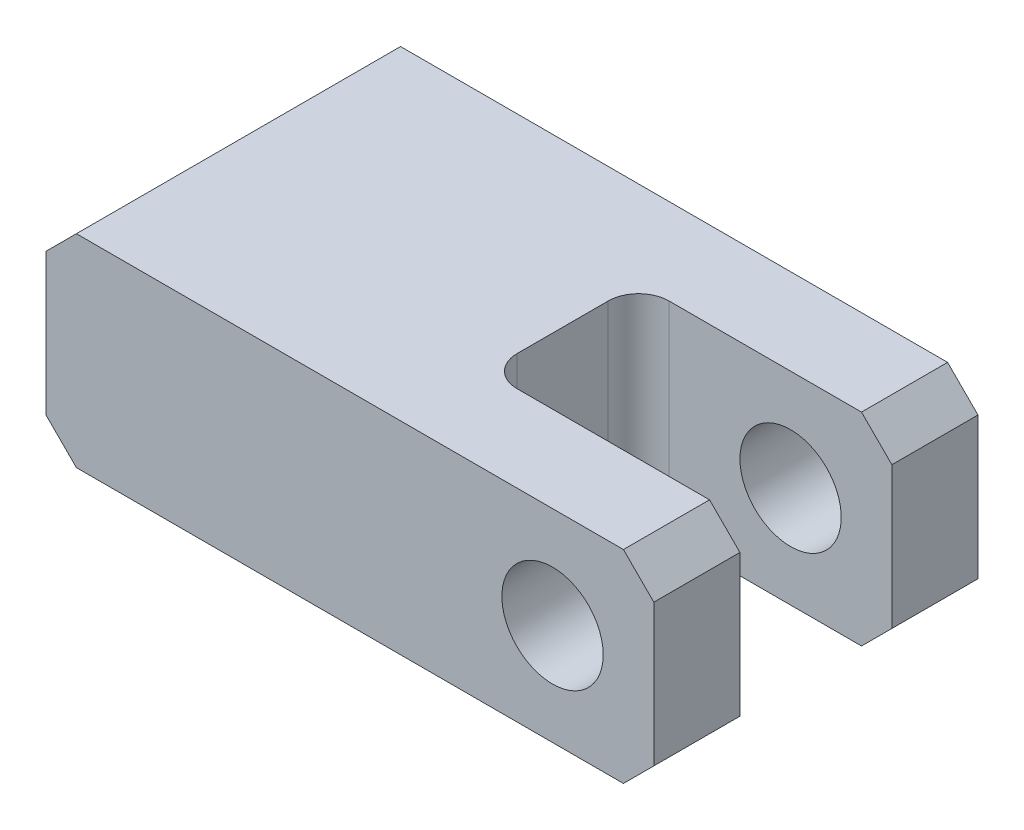
from build123d import *

# Parameters (mm, degrees)
SKETCH1_W             = 60
SKETCH1_H             = 32
BOSS_EXTRUDE1_DEPTH   = 20
SKETCH2_R             = 5
CUT_EXTRUDE1_DEPTH    = 42
CHAMFER1_SIZE         = 3
M6_TAPPED_HOLE1_D     = 5
M6_TAPPED_HOLE1_DEPTH = 15
M6_TAPPED_HOLE1_TIP   = 1.502151548
SKETCH6_W             = 15
SKETCH6_H             = 30
CUT_EXTRUDE2_DEPTH    = 25
FILLET1_R             = 3


with BuildPart() as part:
    # Sketch1 → Boss-Extrude1 (new body)
    with BuildSketch(Plane(origin=(0, 0, 0), x_dir=(1, 0, 0), z_dir=(0, 1, 0))):
        Rectangle(SKETCH1_W, SKETCH1_H)
    extrude(amount=BOSS_EXTRUDE1_DEPTH)

    # Sketch2 → Cut-Extrude1 (cut)
    with BuildSketch(Plane.XY.offset(16)):
        with Locations((20, 10)):
            Circle(SKETCH2_R)
    extrude(amount=-CUT_EXTRUDE1_DEPTH, mode=Mode.SUBTRACT)

    # Chamfer1
    chamfer1_edges = [part.edges().sort_by_distance(p)[0] for p in [
        (30, 20, 0),
        (-30, 20, 0),
        (30, 0, 0),
        (-30, 0, 0),
    ]]
    chamfer(chamfer1_edges, length=CHAMFER1_SIZE)

    # M6 Tapped Hole1
    with Locations(Plane.ZY.offset(30)):
        with Locations((-10, 10), (10, 10)):
            Hole(M6_TAPPED_HOLE1_D / 2, depth=M6_TAPPED_HOLE1_DEPTH)
            with Locations((0, 0, -(M6_TAPPED_HOLE1_DEPTH + M6_TAPPED_HOLE1_TIP / 2))):  # 118° drill point
                Cone(0, M6_TAPPED_HOLE1_D / 2, M6_TAPPED_HOLE1_TIP, mode=Mode.SUBTRACT)

    # Sketch6 → Cut-Extrude2 (cut)
    with BuildSketch(Plane(origin=(30, 0, 0), x_dir=(0, 0, -1), z_dir=(1, 0, 0))):
        with Locations((0, 10)):
            Rectangle(SKETCH6_W, SKETCH6_H)
    extrude(amount=-CUT_EXTRUDE2_DEPTH, mode=Mode.SUBTRACT)

    # Fillet1
    fillet1_edges = [part.edges().sort_by_distance(p)[0] for p in [
        (5, 10, -7.5),
        (5, 10, 7.5),
    ]]
    fillet(fillet1_edges, radius=FILLET1_R)


solid = part.part
